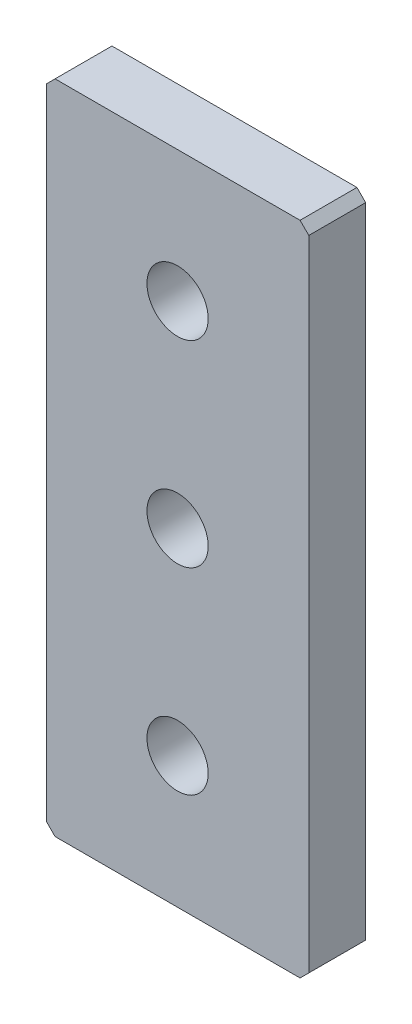
from build123d import *

# Parameters (mm, degrees)
SKETCH_1_W            = 30
SKETCH_1_H            = 75
EXTRUDE_1_DEPTH       = 6.5
HOLE_WIZARD_7_0_7_1_D = 7
CHAMFER_1_SIZE        = 1


with BuildPart() as part:
    # 草图1 → 凸台-拉伸1 (new body)
    with BuildSketch(Plane.XY):
        Rectangle(SKETCH_1_W, SKETCH_1_H)
    extrude(amount=EXTRUDE_1_DEPTH)

    # Ø7.0 (7) 直径孔1 (through all)
    with Locations(Plane.XY.offset(6.5)):
        with Locations((0, 0), (0, -22.5), (0, 22.5)):
            Hole(HOLE_WIZARD_7_0_7_1_D / 2)

    # 倒角1
    chamfer_1_edges = [part.edges().sort_by_distance(p)[0] for p in [
        (15, -37.5, 3.25),
        (-15, -37.5, 3.25),
        (-15, 37.5, 3.25),
        (15, 37.5, 3.25),
    ]]
    chamfer(chamfer_1_edges, length=CHAMFER_1_SIZE)


solid = part.part
